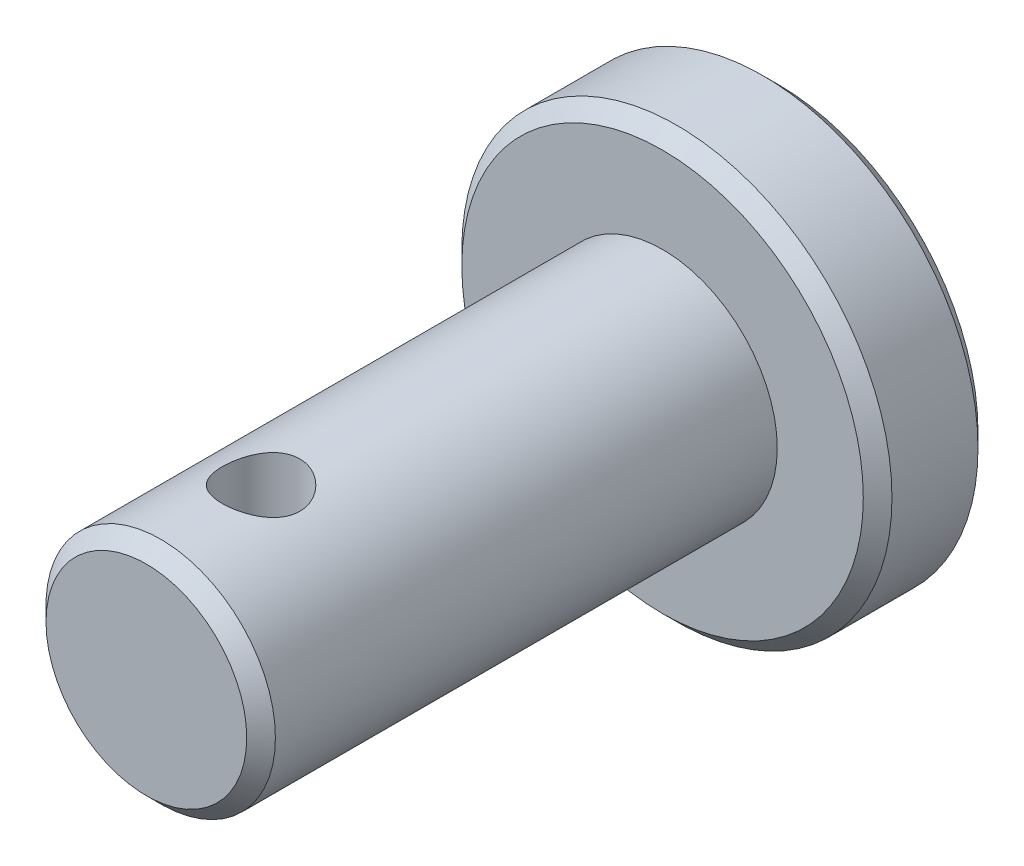
SolidWorks part; units mm, degrees
material "国产6061 "
ref_plane "Front Plane" through (0, 0, 0) normal (0, 0, 1) x (1, 0, 0)
ref_plane "Top Plane" through (0, 0, 0) normal (0, 1, 0) x (1, 0, 0)
ref_plane "Right Plane" through (0, 0, 0) normal (1, 0, 0) x (0, 0, -1)
sketch "Sketch1" plane through (0, 0, 0) normal (0, 0, 1) x (1, 0, 0)
  circle A0 centre (0, 0) radius 4
  dimension "D1" = 8
extrude "Boss-Extrude1" add sketch "Sketch1" along normal blind 18
sketch "Sketch2" plane through (0, 0, 0) normal (0, 0, -1) x (-1, 0, 0)
  circle A0 centre (0, 0) radius 7.5
  dimension "D1" = 15
extrude "Boss-Extrude2" add sketch "Sketch2" along normal blind 4
sketch "Sketch3" plane through (0, 0, 0) normal (0, 1, 0) x (1, 0, 0)
  line L0 (-4, -18) -> (4, -18) construction
  circle A0 centre (0, -14) radius 1.35
  dimension "D1" = 2.7
  dimension "D2" = 4
extrude "Cut-Extrude1" cut sketch "Sketch3" against normal through all both and the other way through all
chamfer "Chamfer1" distance 0.5 angle 45 3 edges at (4, 0, 18) (-7.5, 0, -4) (-7.5, 0, 0)
